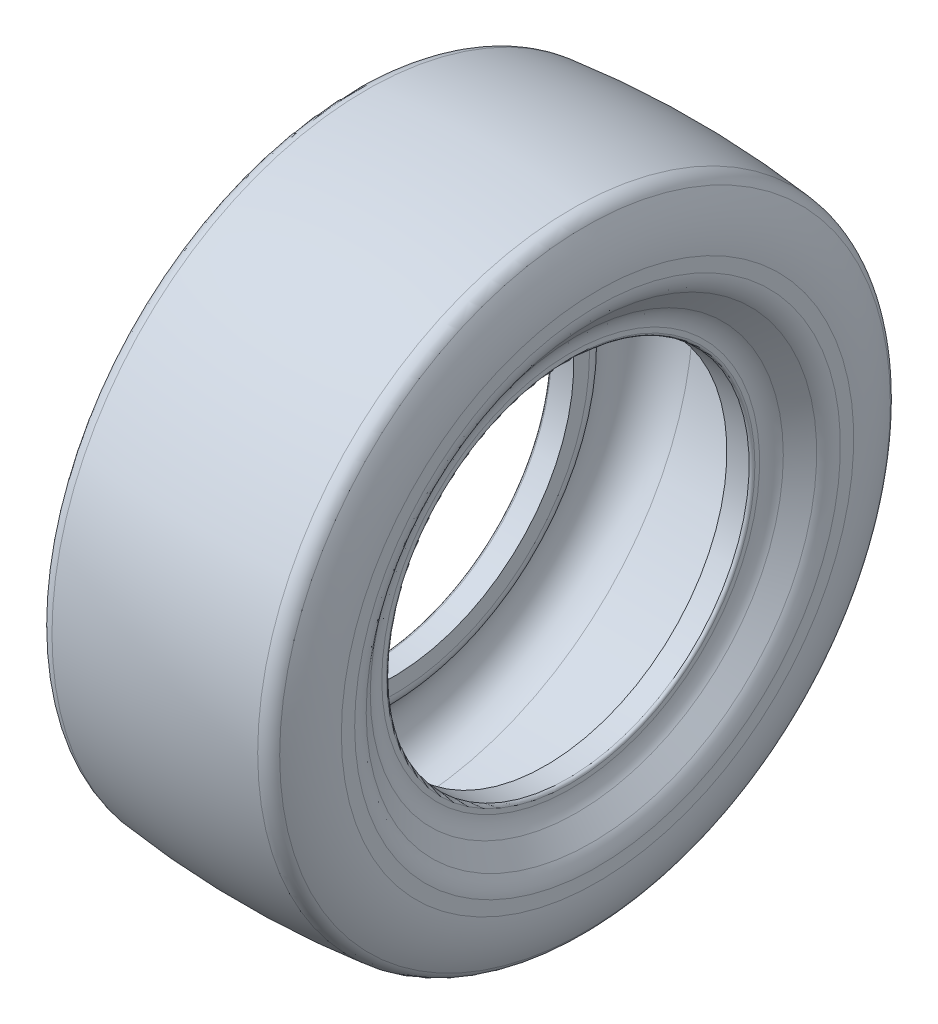
SolidWorks part; units mm, degrees
material "橡胶"
ref_plane "前视基准面" through (0, 0, 0) normal (0, 0, 1) x (1, 0, 0)
ref_plane "上视基准面" through (0, 0, 0) normal (0, 1, 0) x (1, 0, 0)
ref_plane "右视基准面" through (0, 0, 0) normal (1, 0, 0) x (0, 0, -1)
sketch "草图1" plane through (0, 0, 0) normal (0, 0, 1) x (1, 0, 0)
  line L0 (0, 0) -> (32.0071, 0) construction
  line L1 (0, 0) -> (0, 37.2296) construction
  line L2 (-173, 317.5) -> (173, 317.5)
  line L3 (-178, 322.5) -> (-178, 330.7283)
  line L4 (-188.6532, 361.5801) -> (-214.3468, 394.3482)
  line L5 (-225, 425.2) -> (-225, 448.5)
  line L6 (-638.2724, 560) -> (726.2745, 560) construction
  line L7 (225, 425.2) -> (225, 448.5)
  line L8 (188.6532, 361.5801) -> (214.3468, 394.3482)
  line L9 (178, 322.5) -> (178, 330.7283)
  line L10 (-1276.235, -560) -> (1002.5529, -560) construction
  arc A0 (-173, 317.5) -> (-178, 322.5) centre (-173, 322.5) cw
  arc A1 (-178, 330.7283) -> (-188.6532, 361.5801) centre (-228, 330.7283) ccw
  arc A2 (-225, 425.2) -> (-214.3468, 394.3482) centre (-175, 425.2) ccw
  arc A3 (180.0543, 550.0353) -> (-180.0543, 550.0353) centre (0, -1071.7) ccw
  arc A4 (-203.0927, 534.5622) -> (-225, 448.5) centre (-45, 448.5) ccw
  arc A5 (-203.0927, 534.5622) -> (-180.0543, 550.0353) centre (-176.7439, 520.2185) cw
  arc A6 (203.0927, 534.5622) -> (180.0543, 550.0353) centre (176.7439, 520.2185) ccw
  arc A7 (203.0927, 534.5622) -> (225, 448.5) centre (45, 448.5) cw
  arc A8 (225, 425.2) -> (214.3468, 394.3482) centre (175, 425.2) cw
  arc A9 (178, 330.7283) -> (188.6532, 361.5801) centre (228, 330.7283) cw
  arc A10 (173, 317.5) -> (178, 322.5) centre (173, 322.5) ccw
  dimension "D1" = 635
  dimension "D2" = 356
  dimension "D3" = 51.9
  dimension "D4" = 5
  dimension "D10" = 180
  dimension "D11" = 1631.7
  dimension "D12" = 1120
  dimension "D13" = 30
  dimension "D14" = 560
  dimension "D9" = 90
  dimension "D6" = 50
  dimension "D8" = 897
  dimension "D5" = 450
  dimension "D7" = 850.4
revolve "旋转1" add sketch "草图1" angle 360 about L0
sketch "草图3" plane through (0, 0, 0) normal (0, 0, 1) x (1, 0, 0)
  line L0 (0, 0) -> (354.9033, 0) construction
  line L1 (0, 0) -> (0, 249.4368) construction
  line L2 (-134, -317.5) -> (134, -317.5)
  line L3 (-134, -317.5) -> (-134, -344.8136)
  line L4 (-142.6392, -365.8782) -> (-165.2918, -388.8493)
  line L5 (142.6392, -365.8782) -> (165.2918, -388.8493)
  line L6 (134, -317.5) -> (134, -344.8136)
  line L7 (-115.45, -508) -> (115.45, -508)
  arc A0 (-142.6392, -365.8782) -> (-134, -344.8136) centre (-164, -344.8136) ccw
  arc A1 (-165.2918, -388.8493) -> (-115.45, -508) centre (-115.45, -438) ccw
  arc A2 (165.2918, -388.8493) -> (115.45, -508) centre (115.45, -438) cw
  arc A3 (142.6392, -365.8782) -> (134, -344.8136) centre (164, -344.8136) cw
  dimension "D4" = 30
  dimension "D7" = 70
  dimension "D1" = 635
  dimension "D2" = 268
  dimension "D3" = 45.4
  dimension "D5" = 1016
  dimension "D6" = 230.9
revolve "切除-旋转1" cut sketch "草图3" angle 360 about L0
